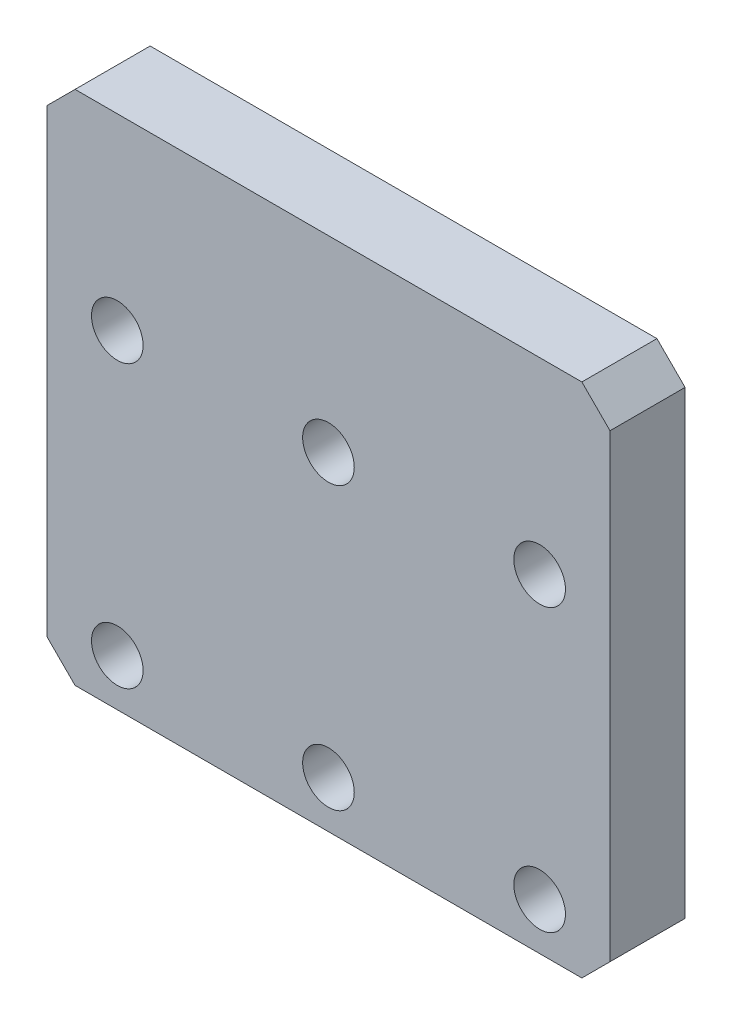
SolidWorks part; units mm, degrees
ref_plane "Front Plane" through (0, 0, 0) normal (0, 0, 1) x (1, 0, 0)
ref_plane "Top Plane" through (0, 0, 0) normal (0, 1, 0) x (1, 0, 0)
ref_plane "Right Plane" through (0, 0, 0) normal (1, 0, 0) x (0, 0, -1)
sketch "Sketch1" plane through (0, 0, 0) normal (0, 0, 1) x (1, 0, 0)
  line L1 (-30, 27.5) -> (30, 27.5)
  line L2 (-30, 27.5) -> (-30, -27.5)
  line L3 (-30, -27.5) -> (30, -27.5)
  line L4 (30, 27.5) -> (30, -27.5)
  line L5 (-30, 27.5) -> (30, -27.5) construction
  line L6 (-30, -27.5) -> (30, 27.5) construction
  point P0 (0, 0)
  dimension "D1" = 60
  dimension "D2" = 55
extrude "Boss-Extrude1" add sketch "Sketch1" along normal blind 8
hole_wizard "Ø5.5 (5.5) Diameter Hole1" positions "Sketch7" profile "Sketch6" hole size "Ø5.5" standard "GB"
sketch "Sketch7" plane through (0, 0, 8) normal (0, 0, 1) x (1, 0, 0)
  point P1 (-22.5, -22.5)
  point P5 (-22.5, 7.5)
  point P9 (0, 7.5)
  point P13 (0, -22.5)
  point P17 (22.5, -22.5)
  point P21 (22.5, 7.5)
sketch "Sketch6" plane through (-22.5, -22.5, 8) normal (1, 0, 0) x (0, -1, 0)
  line L0 (0, 0) -> (0, 8)
  line L1 (0, 8) -> (2.75, 8)
  line L2 (2.75, 8) -> (2.75, 0)
  line L5 (2.75, 0) -> (0, 0)
  line L11 (0, -6.35) -> (0, 107.95) construction
  dimension "通孔孔直径" = 5.5
  dimension "通孔孔深度" = 8
chamfer "Chamfer1" distance 3 angle 45 4 edges at (30, 27.5, 4) (-30, 27.5, 4) (-30, -27.5, 4) (30, -27.5, 4)
